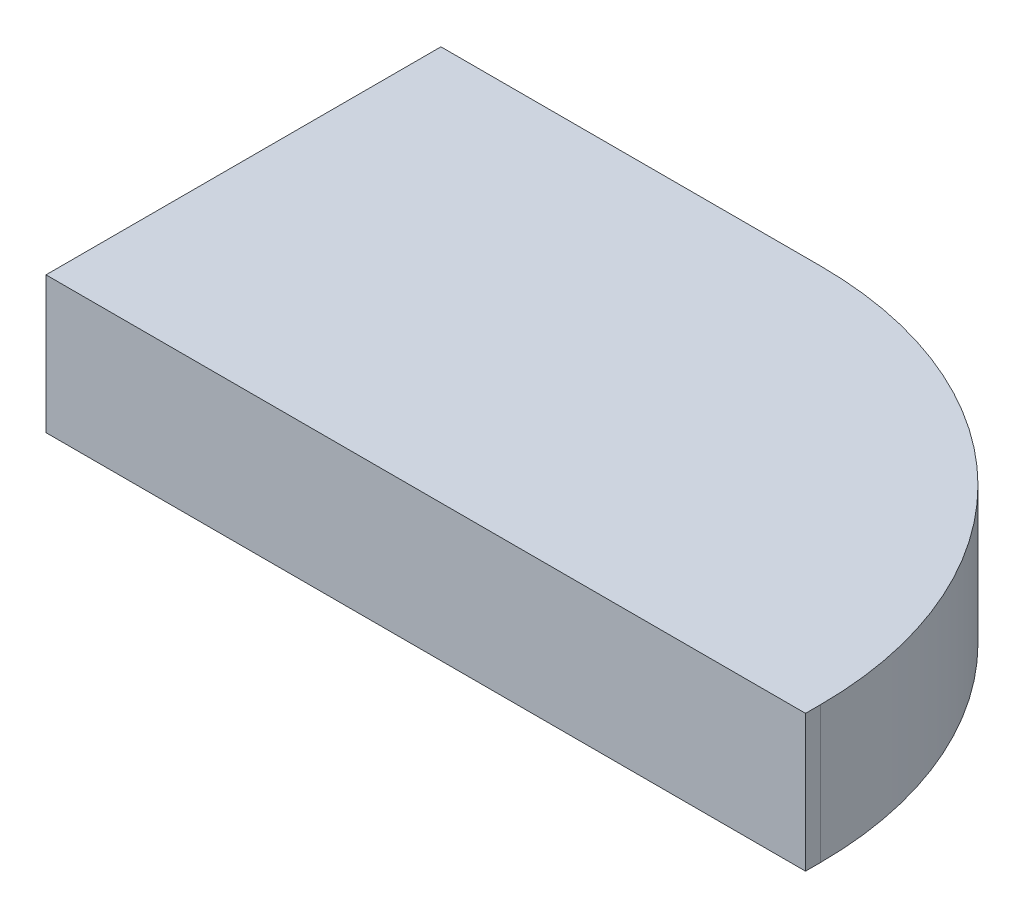
SolidWorks part; units mm, degrees
ref_plane "Front Plane" through (0, 0, 0) normal (0, 0, 1) x (1, 0, 0)
ref_plane "Top Plane" through (0, 0, 0) normal (0, 1, 0) x (1, 0, 0)
ref_plane "Right Plane" through (0, 0, 0) normal (1, 0, 0) x (0, 0, -1)
sketch "Sketch1" plane through (0, 0, 0) normal (0, 1, 0) x (1, 0, 0)
  line L1 (0, 0) -> (25, 0)
  line L2 (0, 0) -> (0, 13)
  line L3 (0, 13) -> (12.5, 13)
  line L4 (25, 0) -> (25, 0.5)
  arc A0 (12.5, 13) -> (25, 0.5) centre (12.5, 0.5) cw
  dimension "D3" = 12.5
  dimension "D1" = 25
  dimension "D2" = 13
extrude "Boss-Extrude1" add sketch "Sketch1" along normal mid plane 4.5
